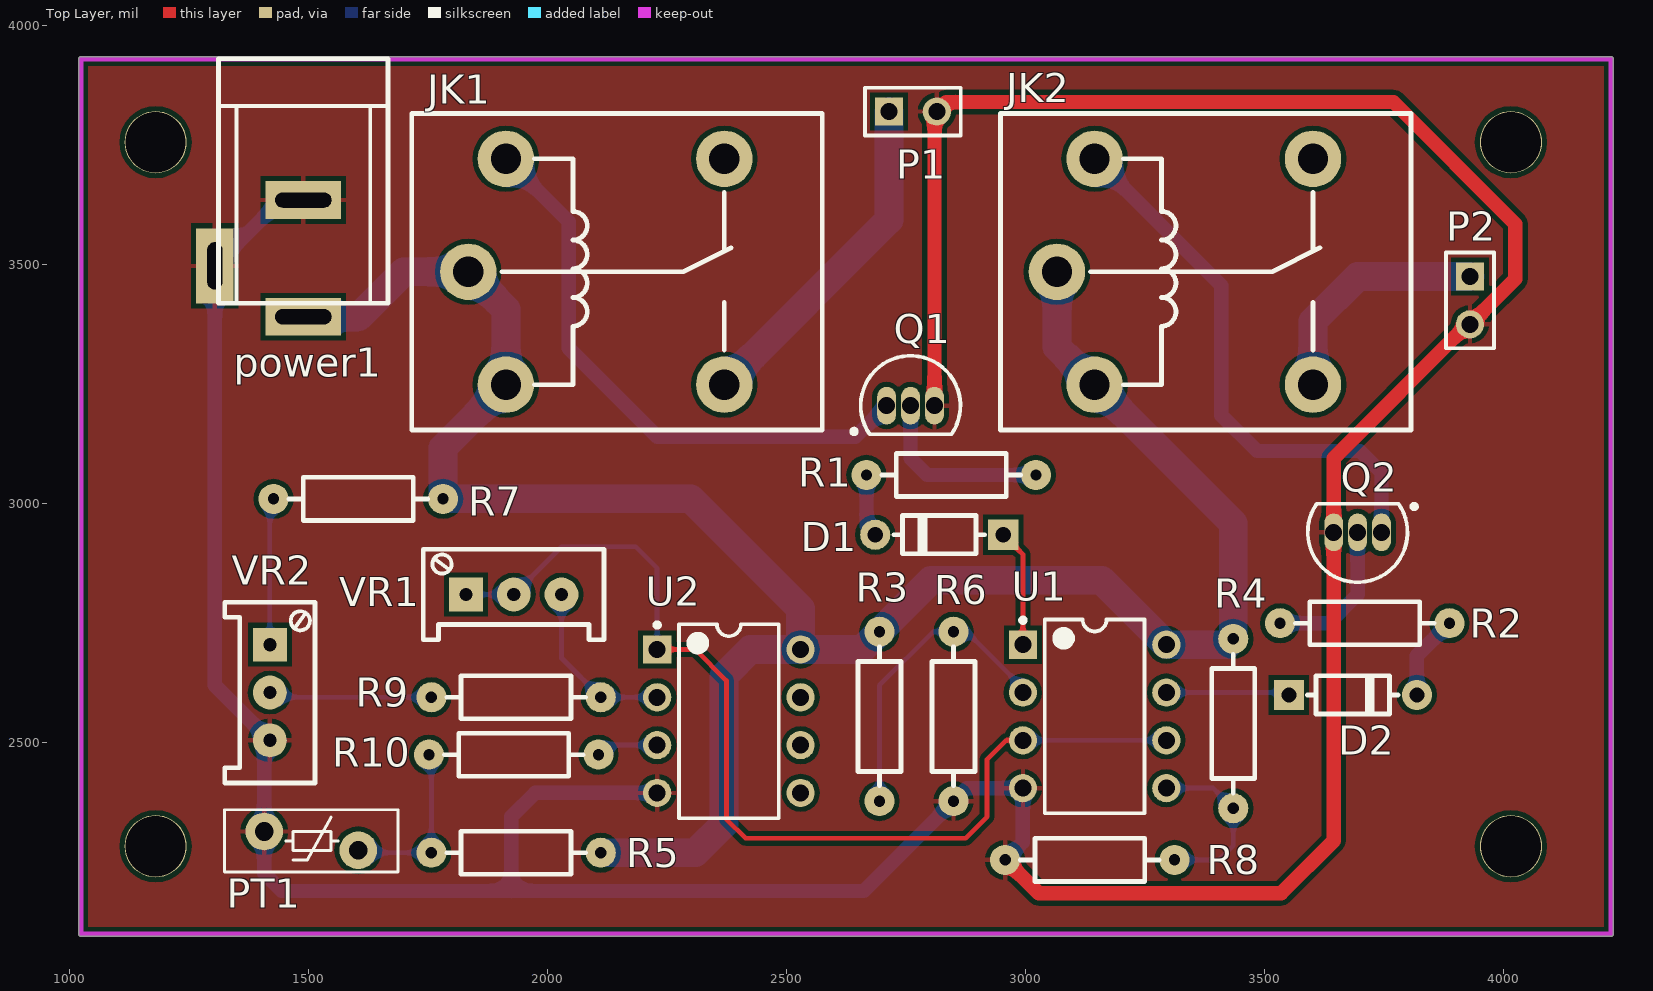
[diagram p0: Top Layer view]
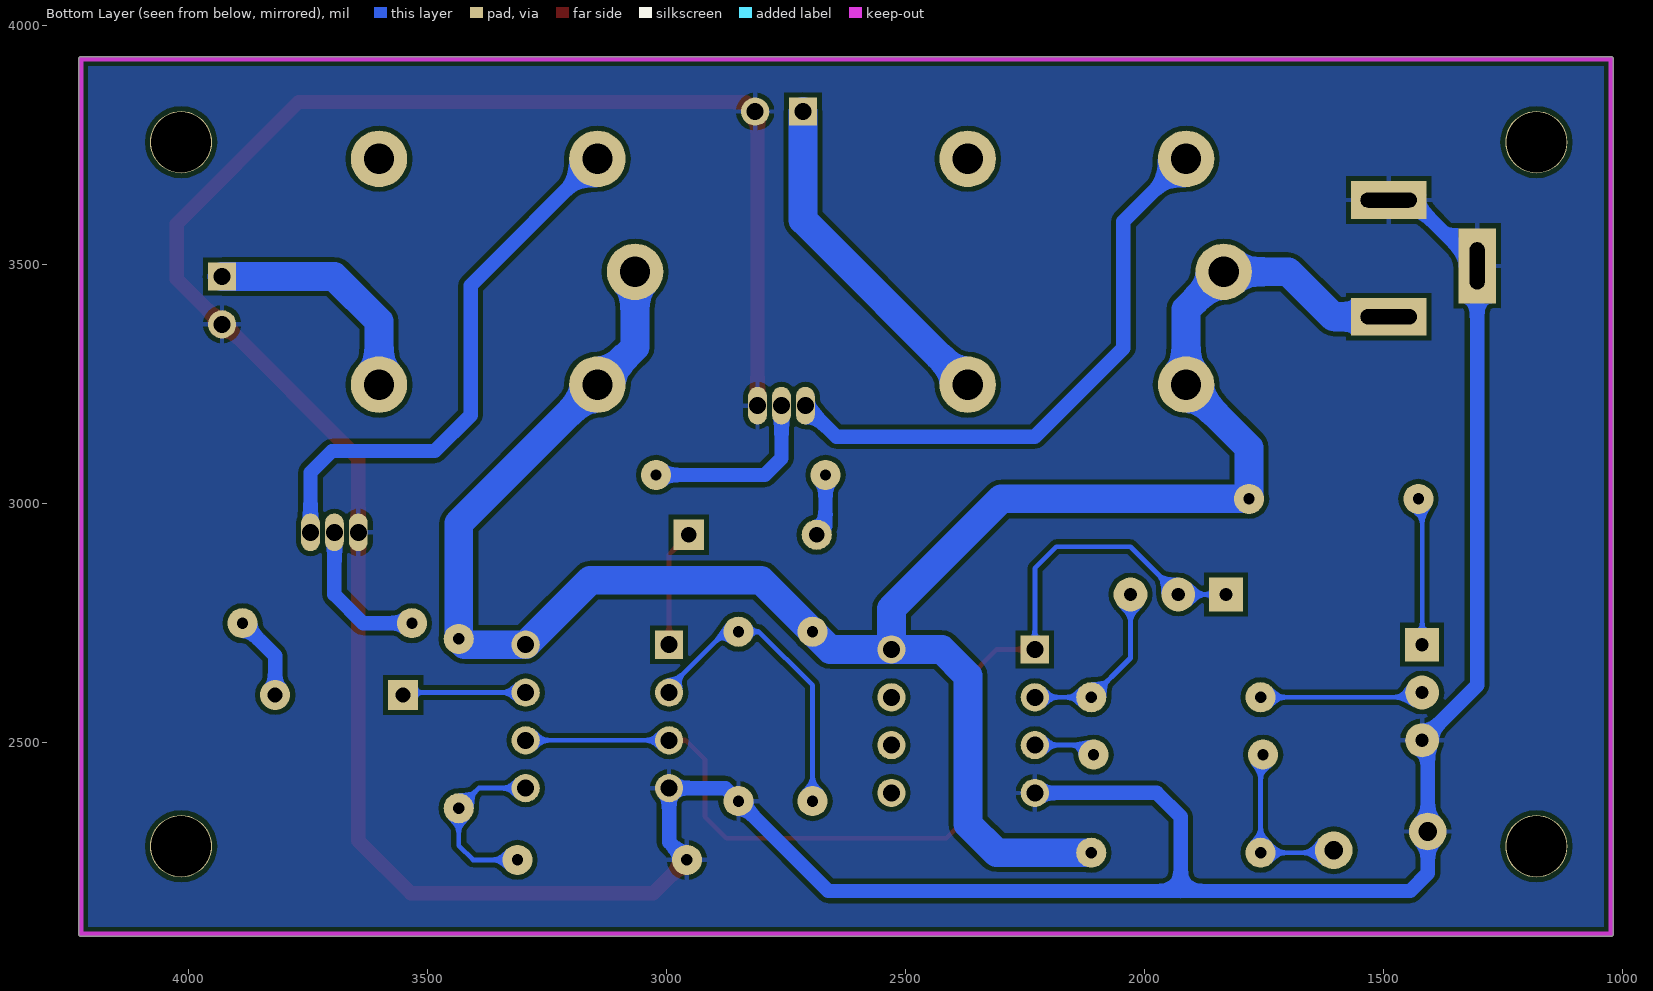
[diagram p1: Bottom Layer view, seen from below]
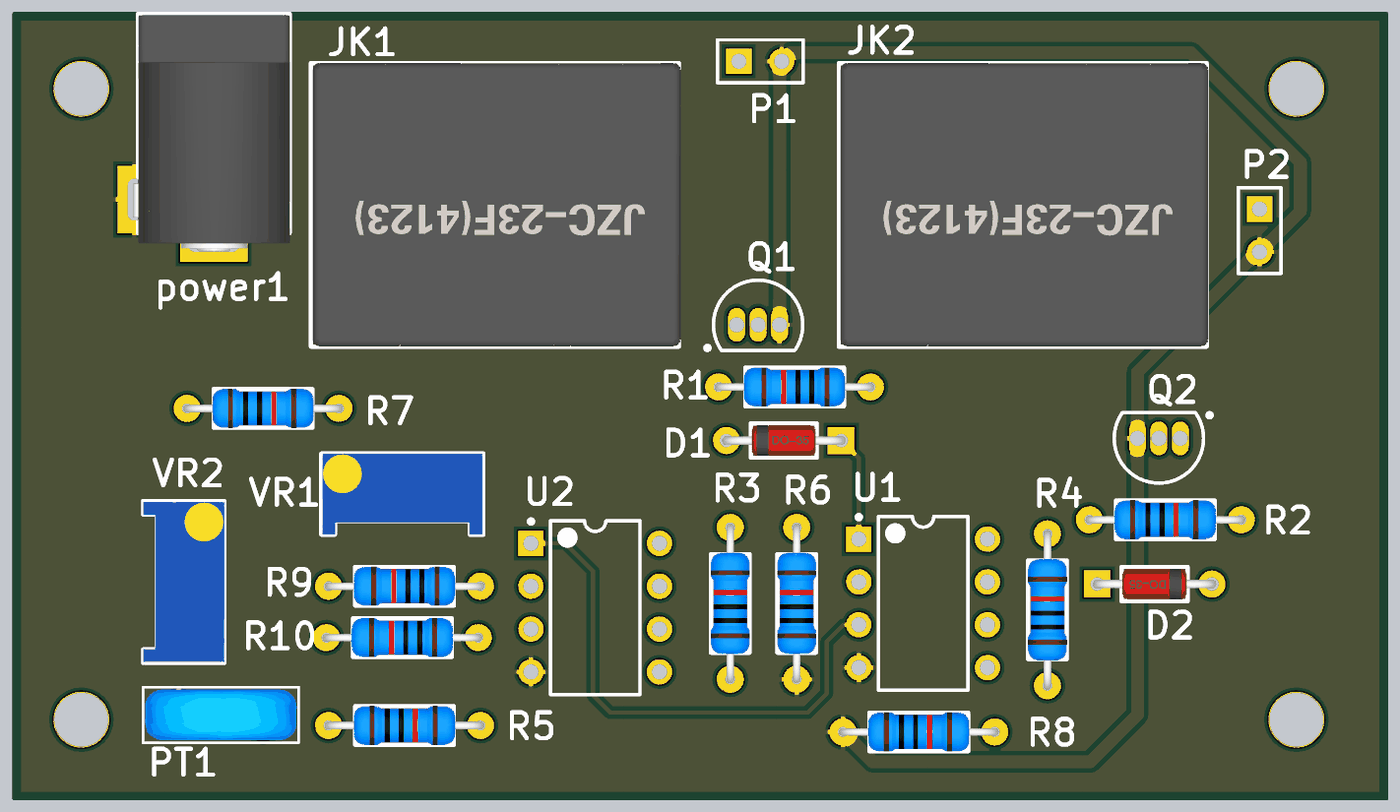
[diagram p2: 3D render of the assembled board from above, using the file's embedded part models]
# Altium PCB MISC84335.PcbDoc
Units mil, origin at the board's own origin, x right, y up, seen from the top; angles counter-clockwise.
Board outline 3210.03 x 1840.03 mil, 2 copper layers (Top Layer, Bottom Layer); 24 components, 20 nets, 75 pads, 0 vias.

## Layer stack, top to bottom (the 12.6 mil dielectric is the usual default, probably not edited)
Top Solder: solder mask 0.4, Solder Resist, Dk 3.5
Top Layer: signal copper 1.4
Dielectric 1: dielectric 12.6, FR-4, Dk 4.8
Bottom Layer: signal copper 1.4
Bottom Solder: solder mask 0.4, Solder Resist, Dk 3.5

## Board outline
1025,2094.99 cw(c1025,2100) 1019.99,2100 1019.99,3930 cw(c1025,3930) 1025,3935.01 4225,3935.01 cw(c4225,3930) 4230.02,3930 4230.02,2100 cw(c4225,2100) 4225,2094.99

## Design rules (kind name [scope] priority, off if disabled: settings)
Clearance [All] p1: gap=10
HoleSize [All] p1: absolutevalues=TRUE maxlimit=1000 minlimit=1 maxpercent=80.000 minpercent=20.000
MinimumSolderMaskSliver [All] p1: minsoldermaskwidth=0
PolygonConnect [All] p1: connectstyle=Relief reliefconductorwidth=10 reliefentries=4 polygonreliefangle="90 Angle" airgapwidth=10
RoutingVias [All] p1: holewidth=28 width=50 viastyle="Through Hole" minholewidth=28 minwidth=50 maxholewidth=28 maxwidth=50
SilkToSilkClearance [All] p1: silktosilkclearance=0
SilkToSolderMaskClearance [IsPad] p1: minsilkscreentomaskgap=0 clearancetoexposedcopper=TRUE
SolderMaskExpansion [All] p1: expansion=4
Width [All] p1: maxlimit=60 minlimit=10 preferedwidth=10
26 further rules are at their usual default settings.

## Components (designator, comment, footprint, x,y, rotation, side; value= is the part's Value field where it differs from the comment)
D1 "1N4148" DO-35 2820,2935 r180 top
D2 "1N4148" DO-35 3685,2600 r0 top
JK1 "JZC-23F(12VDC)" JZC-23F(4123) 1835,3485 r0 top
JK2 "JZC-23F(12VDC)" JZC-23F(4123) 3066.26,3485 r0 top
P1 "风扇" HDR1X2 2715,3820 r0 top
P2 "加热棒" HDR1X2 3930,3475 r270 top
power1 "" DC-005 1490,3390.91 r90 top
PT1 "PT100" "VDR 9D-4.5" 1408.15,2294.68 r0 top
Q1 "NPN" TO-226-AA 2760,3205 r270 top
Q2 "NPN" TO-226-AA 3695,2940 r90 top
R1 "5k" "RS 1/4W" 2845,3060 r180 top
R2 "5k" "RS 1/4W" 3710,2750 r0 top
R3 "10.36k" "RS 1/4W" 2695,2555 r90 top
R4 "11.75k" "RS 1/4W" 3435,2540 r90 top
R5 "2k" "RS 1/4W" 1935,2270 r0 top
R6 "1.64k" "RS 1/4W" 2850,2555 r90 top
R7 "2k" "RS 1/4W" 1605,3010 r0 top
R8 "250R" "RS 1/4W" 3135,2255 r0 top
R9 "1k" "RS 1/4W" 1935,2595 r180 top
R10 "1k" "RS 1/4W" 1930,2475 r180 top
U1 "AD823AN" DIP-8 3145,2555 r0 top
U2 "AD823AN" DIP-8 2380,2545 r0 top
VR1 "100k" 3296W 1930,2810 r0 top
VR2 "200R" 3296W 1420,2605 r270 top

## Footprints (in the part's own frame and the unit in brackets; to place one, negate y for a bottom-side part, rotate by r counter-clockwise, add the part's x,y. Pads: shape width x height; smd on the part's side, far side on the other; paste and mask are expansions set on the pad)
3296W [mm] "Precise Multi-Winding Adjustable Resistor"
  rect 1.8x1.8 hole 0.7: 1(-2.54,0)
  round 1.8 hole 0.7: 2(0,0) 3(2.54,0)
  silkscreen extent -4.8,-2.4 4.8,2.4, body extent -4.75,-2.4 4.75,2.4, height 11.52
DC-005 [mm] "5.5X2.1mm"
  rect 2x4 hole 0.8 slot 3 at 90 deg: 1(0,0) 2(6.2,0)
  rect 4x2 hole 0.8 slot 2.5 at 0 deg: 3(2.7,4.7)
  silkscreen extent 0.72,-4.5 13.7,4.5, body extent -0.4,-4.52 13.65,4.78, height 11.2
DIP-8 [mm] "DIP; 8 Leads; Row Spacing 7.62 mm; Pitch 2.54 mm"
  rect 1.5x1.5 hole 0.9: 1(-3.81,3.81)
  round 1.5 hole 0.9: 2(-3.81,1.27) 3(-3.81,-1.27) 4(-3.81,-3.81) 5(3.81,-3.81) 6(3.81,-1.27) 7(3.81,1.27) 8(3.81,3.81)
  silkscreen extent -3.93,-5.15 2.65,5.23, body extent -3.6,-5.15 3.6,5.15, height 5.08
DO-35 [mm] "1.8*6.8mm(直径，脚距）"
  rect 1.6x1.6 hole 0.8: 1(-3.4,0)
  round 1.6 hole 0.8: 2(3.4,0)
  silkscreen extent -2.41,-1.02 2.41,1.02, body extent -3.65,-0.9 3.65,0.9, height 1.85
HDR1X2 [mm] "Connector; Header; 2 Position"
  rect 1.5x1.5 hole 0.9: 1(0,0)
  round 1.5 hole 0.9: 2(2.54,0)
  silkscreen extent -1.27,-1.27 3.81,1.27
JZC-23F(4123) [mm] "单刀双投"
  round 3 hole 1.6: 1(2,6) 2(2,-6) 3(0,0) 4(13.6,6) 5(13.6,-6)
  silkscreen extent -3,-8.4 18.8,8.4, body extent -2.9,-8.38 18.9,8.42, height 16.1
"RS 1/4W" [mm] "直插色环电阻，脚距9mm，直径2.3mm"
  round 1.6 hole 0.6: 1(-4.5,0) 2(4.5,0)
  silkscreen extent -3.68,-1.14 3.68,1.14, body extent -4.72,-1.16 4.73,1.16, height 2.32
TO-226-AA [mm] "TO, Flat Index; 3 In-Line, Axial Leads; Body Dia. 4.8mm; Leads 0.55 x 0.51 mm (max)"
  oval 2x1 hole 0.9: 1(0,-1.27) 2(0,0) 3(0,1.27)
  silkscreen extent -2.65,-3.13 1.52,2.65, body extent -2.65,-2.66 1.52,2.66, height 5.33
"VDR 9D-4.5" [mm] "压敏电阻9mm*4.5mm(直径*厚度）"
  round 2 hole 1: 1(0,0.5) 2(5,-0.5)
  silkscreen extent -2.11,-1.65 7.11,1.65, body extent -2,-1.5 7,1.5, height 10

## Part data
D1 D2: library part DIO, "Diode"
JK1 JK2: library part JZC-23F(5VDC), "5V单路双控"
P1 P2: library part CON2
power1: library part power2
PT1: library part "Res Varistor"
Q1 Q2: "NPN Bipolar Transistor"
R1 R2 R3 R4 R5 R6 R7 R8 R9 R10: library part RES
U1 U2: library part LM358_2
VR1 VR2: library part RES-V, "Potentiometer"

## Free pads (board coordinates)
  round 129.92 hole 125.98: 0(1181.1,3755.91) 1(1181.1,2283.46) 2(4015.75,3755.91) 3(4015.75,2283.46)

## Nets (pads, with @x,y where several pads share a name; then routed paths per layer and width w, separated by ;. In a path a pad name is that pad's centre, name@x,y a point inside that pad or via, vN(x,y) a via of type N, cw(c..) or ccw(c..) an arc to the next point about the centre after c; other vN are vias at no path point)
+12V: JK1.2 JK1.3 JK2.2 JK2.3 power1.1 R3.2 R4.2 R5.2 R7.2 U1.8 U2.8 | length 4596.3
  Bottom Layer w60: power1.1 1605.91,3390.91 1700,3485 JK1.3 1913.74,3406.26 JK1.2 1782.17,3117.2 R7.2 2300,3010 2530,2780 U2.8 ; R5.2 2310,2270 2370,2330 2370,2640 2425,2695 U2.8 ; JK2.3 3066.26,3327.52 JK2.2 3435,2958.78 R4.2 3422.83,2705 U1.8 3160,2840 2802.83,2840 R3.2 2657.83,2695 U2.8
GND: P1.2 P2.2 power1.2 power1.3 PT1.1 Q1.3 Q2.3 R6.1 R8.1 U1.4 U2.4 VR2.3 | length 8055.3
  Top Layer w30: Q1.3 2810,3815 P1.2 2835,3840 3770,3840 4025,3585 4025,3470 P2.2 3925,3375 3645,3095 Q2.3 3645,2295 3535,2185 3027.83,2185 R8.1
  Bottom Layer w30: power1.2 1442.76,3635 power1.3 1304.96,2620.04 VR2.3 1408.15,2493.15 PT1.1 1408.15,2226.85 1445,2190 1925,2190 ; U2.4 1975,2395 1925,2345 1925,2190 ; R8.1 2995,2292.17 U1.4 2877.17,2405 R6.1 2662.17,2190 1925,2190
NetD1_1: D1.1 U1.1 | length 247
  Top Layer w10: D1.1 2995,2893.86 U1.1
NetD1_2: D1.2 R1.2 | length 132.6
  Bottom Layer w30: R1.2 2667.83,2953.31 D1.2
NetD2_1: D2.1 U1.7 | length 258.2
  Bottom Layer w10: U1.7 3546.14,2605 D2.1
NetD2_2: D2.2 R2.2 | length 178.3
  Bottom Layer w30: D2.2 3818.86,2681.69 R2.2
NetJK1_1: JK1.1 Q1.1 | length 1219.1
  Bottom Layer w30: JK1.1 2045,3589.96 2045,3325 2230,3140 2645,3140 Q1.1
NetJK1_5: JK1.5 P1.1 | length 713.9
  Bottom Layer w60: JK1.5 2715,3593.35 P1.1
NetJK2_1: JK2.1 Q2.1 | length 1155.7
  Bottom Layer w30: JK2.1 3410,3456.22 3410,3185 3485,3110 3700,3110 3745,3065 Q2.1
NetJK2_5: JK2.5 P2.1 | length 499.9
  Bottom Layer w60: JK2.5 3601.69,3381.69 3695,3475 P2.1
NetPT1_2: PT1.2 R5.1 R10.2 | length 362
  Bottom Layer w10: PT1.2 1610,2270 R5.1 1757.83,2470 R10.2
NetQ1_2: Q1.2 R1.1 | length 386.7
  Bottom Layer w30: Q1.2 2760,3095 2795,3060 R1.1
NetQ2_2: Q2.2 R2.1 | length 317
  Bottom Layer w30: R2.1 3635,2750 3695,2810 Q2.2
NetR3_1: R3.1 R6.2 U1.2 | length 647.2
  Bottom Layer w10: R3.1 2695,2620 2807.17,2732.17 R6.2 2877.83,2732.17 2995,2615 U1.2
NetR4_1: R4.1 R8.2 U1.5 | length 370.6
  Bottom Layer w10: U1.5 3392.83,2405 R4.1 3435,2285 3405,2255 R8.2
NetR7_1: R7.1 VR2.1 | length 308.2
  Bottom Layer w10: VR2.1 1420,3002.17 R7.1
NetR9_1: R9.1 U2.2 VR1.3 | length 366.9
  Bottom Layer w10: VR1.3 2030,2677.17 R9.1 U2.2
NetR9_2: R9.2 VR2.2 | length 342
  Bottom Layer w10: VR2.2 1430,2595 R9.2
NetR10_1: R10.1 U2.3 | length 131.1
  Bottom Layer w10: R10.1 2127.17,2495 U2.3
NetU1_3: U1.3 U1.6 U2.1 VR1.1 VR1.2 | length 2183.8
  Top Layer w10: U2.1 2310,2695 2375,2630 2375,2340 2415,2300 2875,2300 2920,2345 2920,2465 2960,2505 U1.3
  Bottom Layer w10: VR1.1 VR1.2 2030,2910 2185,2910 2230,2865 U2.1 ; U1.3 U1.6
pads on no net: JK1.4 JK2.4 U2.5 U2.6 U2.7

## Polygon pours and split planes (outlines as drawn)
GND on Top Layer "D" (solid, remove dead copper, pour order 0): 865,4015 880,4000 4440,4000 4440,2155 4310,2025 4295,2010 895,2010
GND on Bottom Layer "D" (solid, remove dead copper, pour order 2): 925,4050 4270,4050 4280,4060 4450,3890 4450,1900 1045,1900 930,2015

## Keep-outs
Keep-Out Layer:
  lines w10: 1025,3905 1025,3930 1325,3930 ; 1025,3920 1025,2100 4225,2100 4225,3930 1295,3930